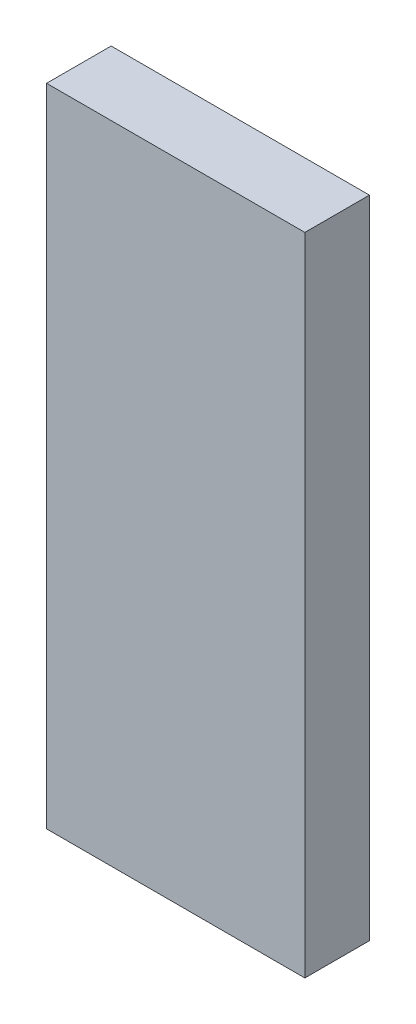
SolidWorks part; units mm, degrees
material "Q235B"
ref_plane "Front Plane" through (0, 0, 0) normal (0, 0, 1) x (1, 0, 0)
ref_plane "Top Plane" through (0, 0, 0) normal (0, 1, 0) x (1, 0, 0)
ref_plane "Right Plane" through (0, 0, 0) normal (1, 0, 0) x (0, 0, -1)
sketch "Sketch1" plane through (0, 0, 0) normal (0, 0, 1) x (1, 0, 0)
  line L1 (0, 0) -> (120, 0)
  line L2 (0, 0) -> (0, 300)
  line L3 (0, 300) -> (120, 300)
  line L4 (120, 0) -> (120, 300)
  dimension "D1" = 300
  dimension "D2" = 120
extrude "Boss-Extrude1" add sketch "Sketch1" along normal blind 30
